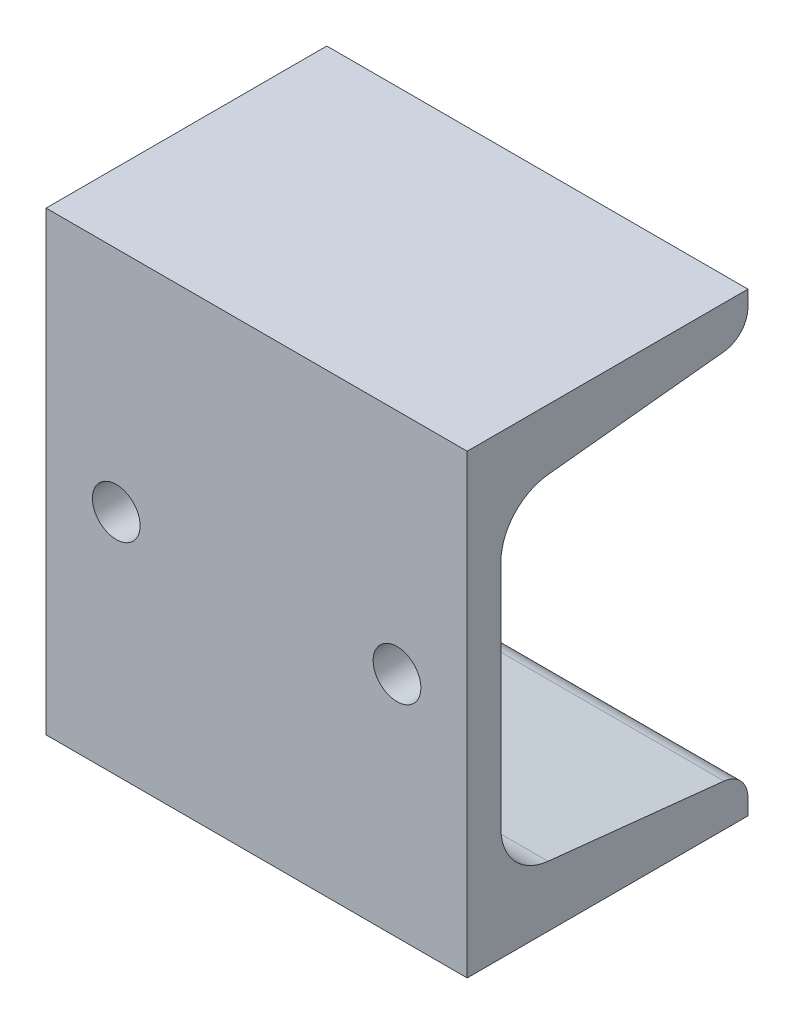
from build123d import *

# Parameters (mm, degrees)
MEMBER_C_6_5_1_DEPTH = 60
HOLE_WIZARD_M8_1_D   = 6.8


with BuildPart() as part:
    # Sketch11 → Member C _ 6.5_1 (new body)
    with BuildSketch(Plane(origin=(0, 0, 0), x_dir=(0, 0, -1), z_dir=(1, 0, 0))):
        with BuildLine():
            Line((40, 65), (0, 65))
            Line((0, 65), (0, 0))
            Line((0, 0), (40, 0))
            Line((40, 0), (40, 2.228630091))
            ThreePointArc((40, 2.228630091), (39.023950337, 4.771326395), (36.59720816, 6.007813293))
            Line((36.59720816, 6.007813293), (11.516036525, 8.643950658))
            ThreePointArc((11.516036525, 8.643950658), (6.726413809, 11.084385325), (4.8, 16.102864873))
            Line((4.8, 16.102864873), (4.8, 48.897135127))
            ThreePointArc((4.8, 48.897135127), (6.726413809, 53.915614675), (11.516036525, 56.356049342))
            Line((11.516036525, 56.356049342), (36.59720816, 58.992186707))
            ThreePointArc((36.59720816, 58.992186707), (39.023950337, 60.228673605), (40, 62.771369909))
            Line((40, 62.771369909), (40, 65))
        make_face()
    extrude(amount=MEMBER_C_6_5_1_DEPTH)

    # M8 螺纹孔1 (through all)
    with Locations(Plane(origin=(10, 32.5, 0), x_dir=(1, 0, 0), z_dir=(0, 0, 1))):
        with Locations((0, 0), (40, 0)):
            Hole(HOLE_WIZARD_M8_1_D / 2)


solid = part.part
